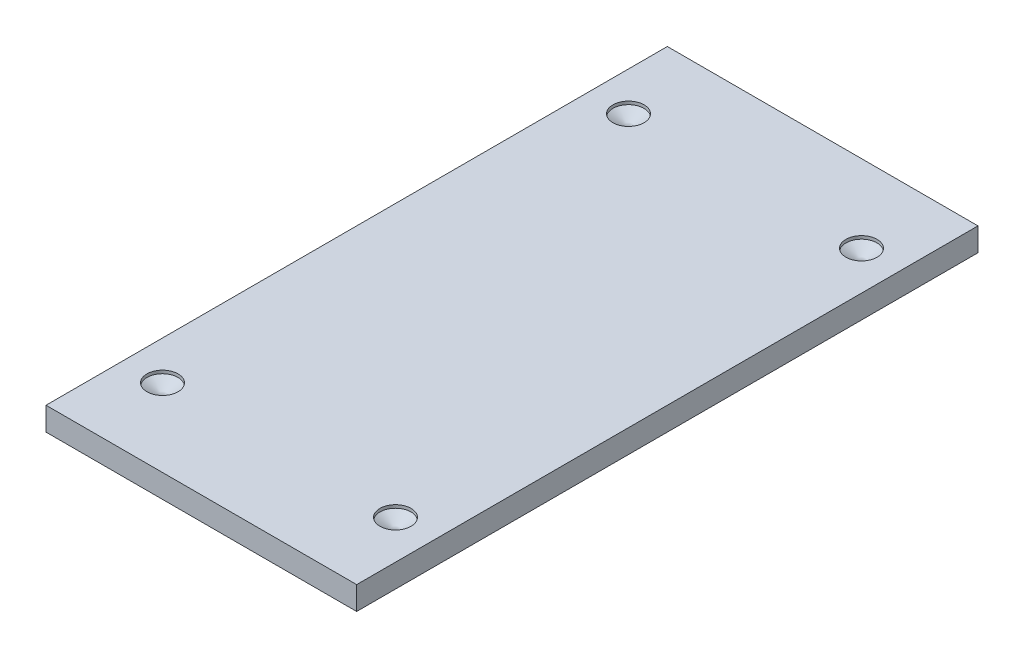
SolidWorks part; units mm, degrees
ref_plane "Front Plane" through (0, 0, 0) normal (0, 0, 1) x (1, 0, 0)
ref_plane "Top Plane" through (0, 0, 0) normal (0, 1, 0) x (1, 0, 0)
ref_plane "Right Plane" through (0, 0, 0) normal (1, 0, 0) x (0, 0, -1)
sketch "Sketch1" plane through (0, 0, 0) normal (0, 1, 0) x (1, 0, 0)
  line L1 (-100, 200) -> (100, 200)
  line L2 (-100, 200) -> (-100, -200)
  line L3 (-100, -200) -> (100, -200)
  line L4 (100, 200) -> (100, -200)
  line L5 (-100, 200) -> (100, -200) construction
  line L6 (-100, -200) -> (100, 200) construction
  point P0 (0, 0)
  dimension "D1" = 200
  dimension "D2" = 400
extrude "Boss-Extrude1" add sketch "Sketch1" along normal blind 15
sketch "Sketch2" plane through (0, 15, 0) normal (0, 1, 0) x (1, 0, 0)
  line L1 (-75, -150) -> (75, -150) construction
  line L2 (-75, -150) -> (-75, 150) construction
  line L3 (-75, 150) -> (75, 150) construction
  line L4 (75, -150) -> (75, 150) construction
  line L5 (-75, -150) -> (75, 150) construction
  line L6 (-75, 150) -> (75, -150) construction
  point P0 (0, 0)
  dimension "D1" = 150
  dimension "D2" = 300
hole_wizard "Ø20.0 (20) Diameter Hole1" positions "Sketch3" profile "Sketch4" hole size "Ø20.0" standard "GB"
sketch "Sketch3" plane through (0, 15, 0) normal (0, 1, 0) x (1, 0, 0)
  point P0 (-75, 150)
  point P3 (-75, -150)
  point P6 (75, -150)
  point P9 (75, 150)
sketch "Sketch4" plane through (-75, 15, -150) normal (1, 0, 0) x (0, 0, 1)
  line L0 (0, 0) -> (0, 8.0086)
  line L1 (0, 8.0086) -> (10, 2)
  line L2 (10, 2) -> (10, 0)
  line L5 (10, 0) -> (0, 0)
  line L10 (0, 8.0086) -> (-10, 2) construction
  line L11 (0, -6.35) -> (0, 107.95) construction
  dimension "孔直径" = 20
  dimension "孔深度" = 2
  dimension "导头角度" = 118
